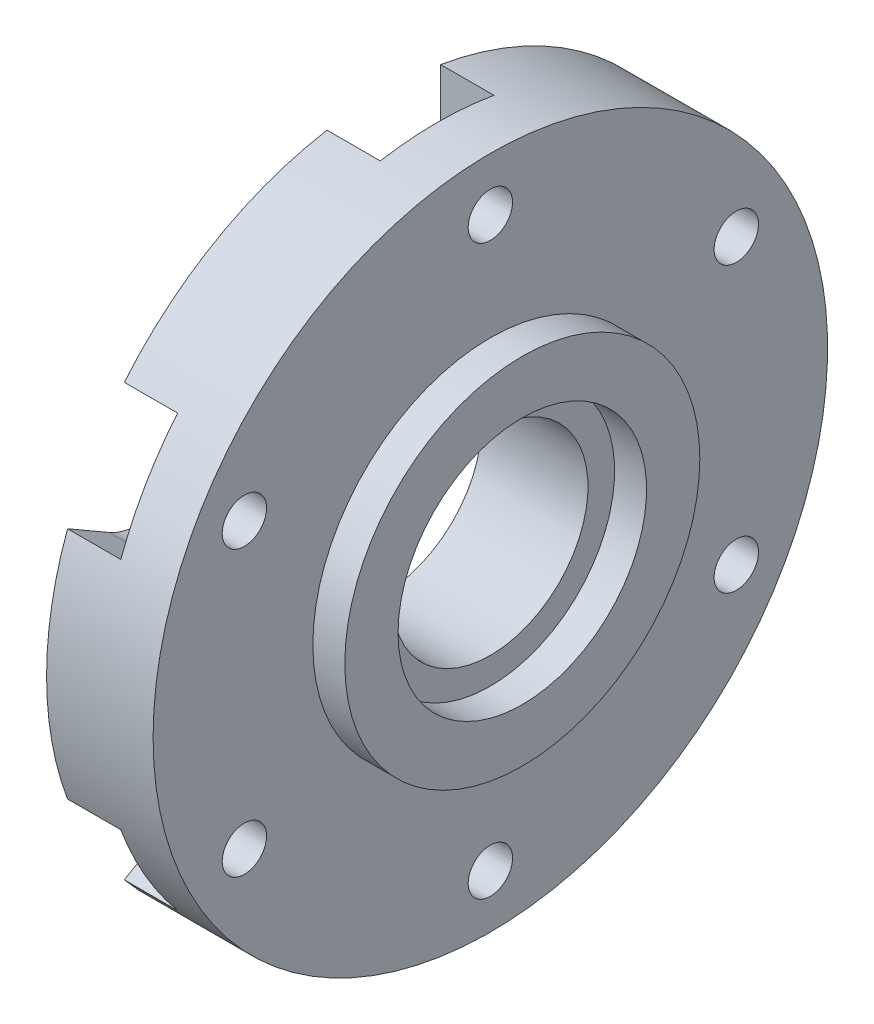
SolidWorks part; units mm, degrees
material "普通碳钢"
ref_plane "前视基准面" through (0, 0, 0) normal (0, 0, 1) x (1, 0, 0)
ref_plane "上视基准面" through (0, 0, 0) normal (0, 1, 0) x (1, 0, 0)
ref_plane "右视基准面" through (0, 0, 0) normal (1, 0, 0) x (0, 0, -1)
sketch "草图1" plane through (0, 0, 0) normal (0, 0, 1) x (1, 0, 0)
  line L0 (0, 0) -> (0, 290.7532) construction
  line L1 (0, 0) -> (356.4696, 0) construction
  line L2 (0, 0) -> (0, 95)
  line L3 (0, 95) -> (30, 95)
  line L4 (30, 95) -> (30, 50)
  line L5 (30, 50) -> (39, 50)
  line L6 (39, 50) -> (39, 35)
  line L7 (39, 35) -> (30, 35)
  line L8 (30, 35) -> (30, 0)
  line L9 (30, 0) -> (0, 0)
  dimension "D1" = 190
  dimension "D2" = 100
  dimension "D3" = 15
  dimension "D4" = 30
  dimension "D5" = 9
revolve "旋转1" add sketch "草图1" angle 360 about L1
sketch "草图2" plane through (0, 0, 0) normal (-1, 0, 0) x (0, 0, 1)
  line L0 (0, 0) -> (0, 80) construction
  circle A0 centre (0, 80) radius 6.25
  dimension "D2" = 12.5
  dimension "D1" = 80
extrude "切除-拉伸1" cut sketch "草图2" against normal through all
pattern_circular "阵列(圆周)1" count 6 over 360 about axis through (0, 0, 0) along (1, 0, 0) of "切除-拉伸1"
sketch "草图3" plane through (0, 0, 0) normal (-1, 0, 0) x (0, 0, 1)
  circle A0 centre (0, 0) radius 27.5
  dimension "D1" = 55
extrude "切除-拉伸2" cut sketch "草图3" against normal through all
sketch "草图6" plane through (0, 0, 0) normal (-1, 0, 0) x (0, 0, 1)
  line L0 (0, 0) -> (0, 106.2432) construction
  line L1 (-16, 80) -> (-16, 93.6429)
  line L2 (16, 80) -> (16, 93.6429)
  circle A0 centre (0, 0) radius 95 construction
  arc A1 (16, 93.6429) -> (-16, 93.6429) centre (0, 0) ccw
  arc A2 (-16, 80) -> (16, 80) centre (0, 80) ccw
  dimension "D1" = 32
extrude "切除-拉伸3" cut sketch "草图6" against normal blind 15
pattern_circular "阵列(圆周)2" count 6 over 360 about axis through (0, 0, 0) along (1, 0, 0) of "切除-拉伸3"
sketch "草图7" plane through (0, 0, 0) normal (-1, 0, 0) x (0, 0, 1)
  line L0 (0, 0) -> (0, 97.7609) construction
  line L1 (0, 0) -> (40, 69.282) construction
  dimension "D1" = 30
  dimension "D2" = 80
hole_wizard "M12 螺纹孔1" positions "3D草图2" profile "草图8" tap size "M12" standard "GB"
sketch3d "3D草图2"
  point P0 (0, 69.282, 40)
sketch "草图8" plane through (0, 69.282, 40) normal (0, 1, 0) x (0, 0, 1)
  line L0 (0, 0) -> (0, 21.0644)
  line L1 (0, 21.0644) -> (5.1, 18)
  line L2 (5.1, 18) -> (5.1, 0)
  line L5 (5.1, 0) -> (0, 0)
  line L10 (0, 21.0644) -> (-5.1, 18) construction
  line L11 (0, -6.35) -> (0, 107.95) construction
  dimension "螺纹孔钻头直径" = 10.2
  dimension "螺纹孔钻头深度" = 18
  dimension "导头角度" = 118
cosmetic thread "孔螺蚊线1" parameters "D1"=15, "D2"=12
pattern_circular "阵列(圆周)3" count 6 over 360 about axis through (0, 0, 0) along (1, 0, 0) of "M12 螺纹孔1"
